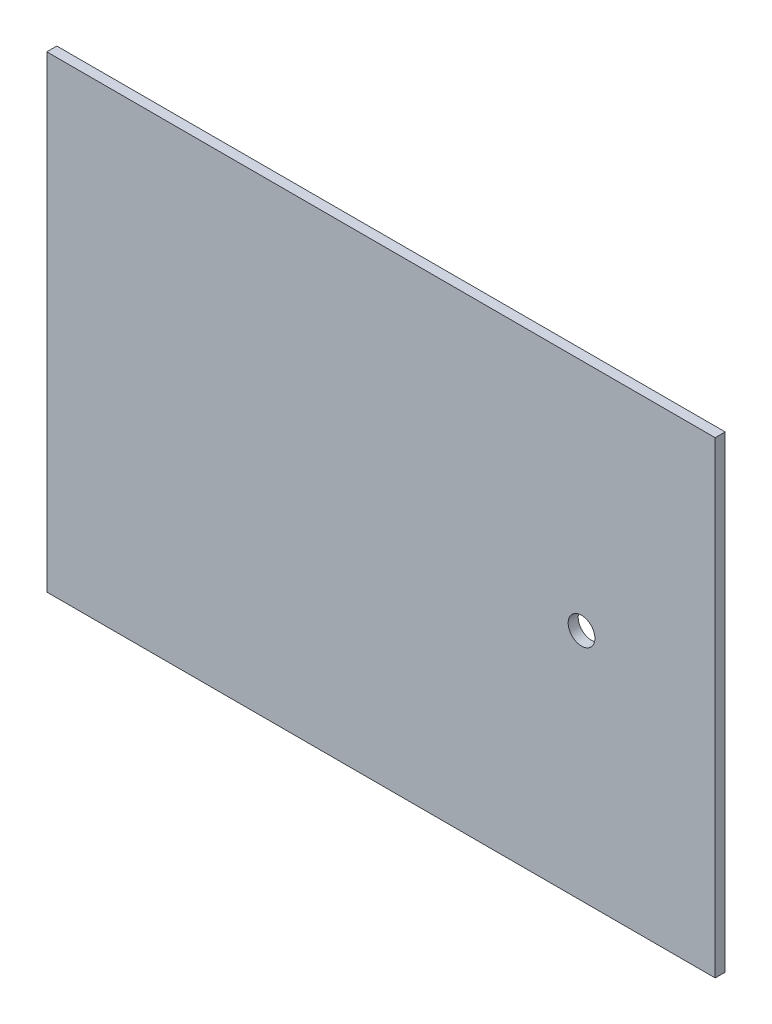
from build123d import *

# Parameters (mm, degrees)
SKETCH_1_W          = 200
SKETCH_1_H          = 140
EXTRUDE_1_DEPTH     = 1.5
SKETCH_2_R          = 4
CUT_EXTRUDE_1_DEPTH = 11.5


with BuildPart() as part:
    # 草图1 → 凸台-拉伸1 (new, symmetric)
    with BuildSketch(Plane.XY):
        Rectangle(SKETCH_1_W, SKETCH_1_H)
    extrude(amount=EXTRUDE_1_DEPTH, both=True)

    # 草图2 → 切除-拉伸1 (cut, symmetric)
    with BuildSketch(Plane.XY):
        with Locations((60, 0)):
            Circle(SKETCH_2_R)
    extrude(amount=CUT_EXTRUDE_1_DEPTH, both=True, mode=Mode.SUBTRACT)


solid = part.part
